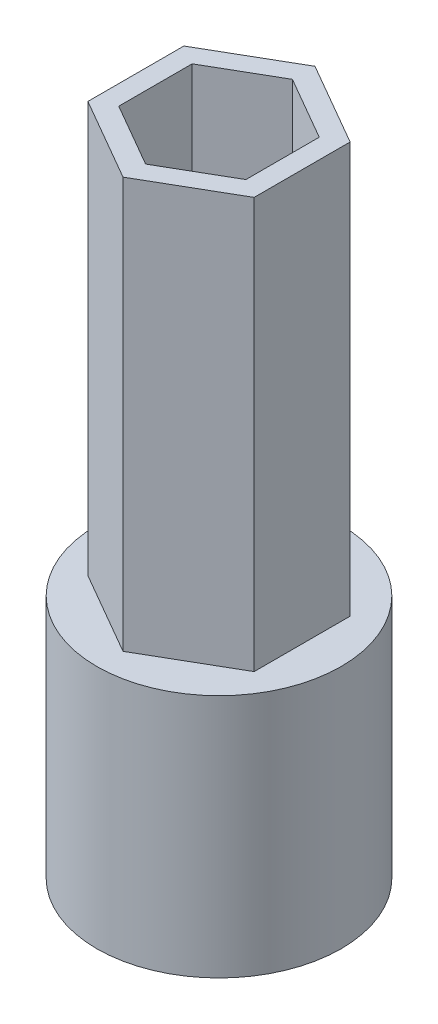
SolidWorks part; units mm, degrees
material "铝"
ref_plane "Front Plane" through (0, 0, 0) normal (0, 0, 1) x (1, 0, 0)
ref_plane "Top Plane" through (0, 0, 0) normal (0, 1, 0) x (1, 0, 0)
ref_plane "Right Plane" through (0, 0, 0) normal (1, 0, 0) x (0, 0, -1)
ref_plane "Plane1" through (0, 13.4, 0) normal (0, 1, 0) x (1, 0, 0)
sketch "Sketch2" plane through (0, 13.4, 0) normal (0, 1, 0) x (1, 0, 0)
  line L1 (0, 1.963) -> (-1.7, 0.9815)
  line L2 (-1.7, 0.9815) -> (-1.7, -0.9815)
  line L3 (-1.7, -0.9815) -> (0, -1.963)
  line L4 (0, -1.963) -> (1.7, -0.9815)
  line L5 (1.7, -0.9815) -> (1.7, 0.9815)
  line L6 (1.7, 0.9815) -> (0, 1.963)
  circle A0 centre (0, 0) radius 1.7 construction
  dimension "D1" = 3.4
sketch "Sketch1" plane through (0, 0, 0) normal (0, 1, 0) x (1, 0, 0)
  arc A0 (0, 2.5) -> (-2.1651, 1.25) centre (0, 0) ccw
  arc A1 (-2.1651, 1.25) -> (-2.1651, -1.25) centre (0, 0) ccw
  arc A2 (-2.1651, -1.25) -> (0, -2.5) centre (0, 0) ccw
  arc A3 (0, -2.5) -> (2.1651, -1.25) centre (0, 0) ccw
  arc A4 (2.1651, -1.25) -> (2.1651, 1.25) centre (0, 0) ccw
  arc A5 (2.1651, 1.25) -> (0, 2.5) centre (0, 0) ccw
  dimension "D1" = 5
extrude "Boss-Extrude3" add sketch "Sketch1" along normal blind 5
extrude "Boss-Extrude4" add sketch "Sketch2" against normal up to surface (8.4 mm away) up to face at (0, 5, 2.5)
shell "Shell1" thickness 0.4
